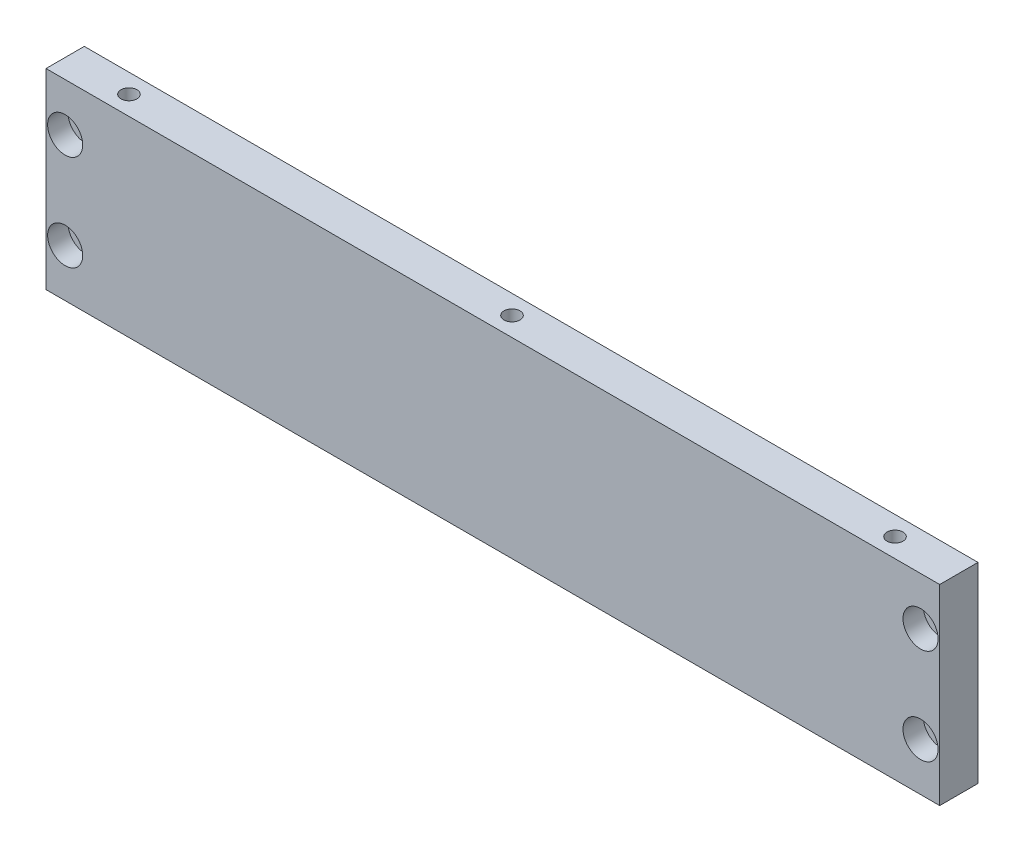
SolidWorks part; units mm, degrees
ref_plane "前视" through (0, 0, 0) normal (0, 0, 1) x (1, 0, 0)
ref_plane "上视" through (0, 0, 0) normal (0, 1, 0) x (1, 0, 0)
ref_plane "右视" through (0, 0, 0) normal (1, 0, 0) x (0, 0, -1)
sketch "草图1" plane through (0, 0, 0) normal (0, 0, 1) x (1, 0, 0)
  line L1 (0, 0) -> (280, 0)
  line L2 (0, 0) -> (0, -60)
  line L3 (0, -60) -> (280, -60)
  line L4 (280, 0) -> (280, -60)
  dimension "D1" = 280
  dimension "D2" = 60
extrude "凸台-拉伸1" add sketch "草图1" along normal blind 12
hole_wizard "M6 螺纹孔1" positions "草图3" profile "草图2" tap size "M6" standard "ISO"
sketch "草图3" plane through (0, 0, 0) normal (0, 1, 0) x (1, 0, 0)
  point P0 (260, -6)
  point P3 (140, -6)
  point P6 (20, -6)
sketch "草图2" plane through (260, 0, 6) normal (1, 0, 0) x (0, 0, 1)
  line L0 (0, 0) -> (0, 16.5022)
  line L1 (0, 16.5022) -> (2.5, 15)
  line L2 (2.5, 15) -> (2.5, 0)
  line L5 (2.5, 0) -> (0, 0)
  line L10 (0, 16.5022) -> (-2.5, 15) construction
  line L11 (0, -6.35) -> (0, 107.95) construction
  dimension "螺纹孔钻头直径" = 5
  dimension "螺纹孔钻头深度" = 15
  dimension "导头角度" = 118
cosmetic thread "孔螺蚊线1"
cosmetic thread "孔螺蚊线2"
cosmetic thread "孔螺蚊线3"
hole_wizard "M6 螺纹孔2" positions "草图5" profile "草图4" tap size "M6" standard "ISO"
sketch "草图5" plane through (0, -60, 0) normal (0, -1, 0) x (-1, 0, 0)
  point P0 (-260, -6)
  point P3 (-140, -6)
  point P6 (-20, -6)
sketch "草图4" plane through (260, -60, 6) normal (1, 0, 0) x (0, 0, -1)
  line L0 (0, 0) -> (0, 16.5022)
  line L1 (0, 16.5022) -> (2.5, 15)
  line L2 (2.5, 15) -> (2.5, 0)
  line L5 (2.5, 0) -> (0, 0)
  line L10 (0, 16.5022) -> (-2.5, 15) construction
  line L11 (0, -6.35) -> (0, 107.95) construction
  dimension "螺纹孔钻头直径" = 5
  dimension "螺纹孔钻头深度" = 15
  dimension "导头角度" = 118
cosmetic thread "孔螺蚊线4"
cosmetic thread "孔螺蚊线5"
cosmetic thread "孔螺蚊线6"
hole_wizard "M6 六角凹头螺钉的柱形沉头孔1" positions "草图7" profile "草图6" counterbore size "M6" standard "ISO" end condition through all
sketch "草图7" plane through (0, 0, 12) normal (0, 0, 1) x (1, 0, 0)
  point P0 (274, -45)
  point P3 (274, -15)
  point P6 (6, -45)
  point P9 (6, -15)
sketch "草图6" plane through (274, -45, 12) normal (1, 0, 0) x (0, -1, 0)
  line L0 (0, 0) -> (0, 12)
  line L1 (0, 12) -> (3.3, 12)
  line L3 (3.3, 12) -> (3.3, 6.4)
  line L4 (3.3, 6.4) -> (5.5, 6.4)
  line L5 (5.5, 6.4) -> (5.5, 0)
  line L7 (5.5, 0) -> (0, 0)
  line L11 (0, -6.35) -> (0, 107.95) construction
  dimension "通孔孔直径" = 6.6
  dimension "通孔孔深度" = 12
  dimension "柱形沉头孔直径" = 11
  dimension "柱形沉头孔深度" = 6.4
